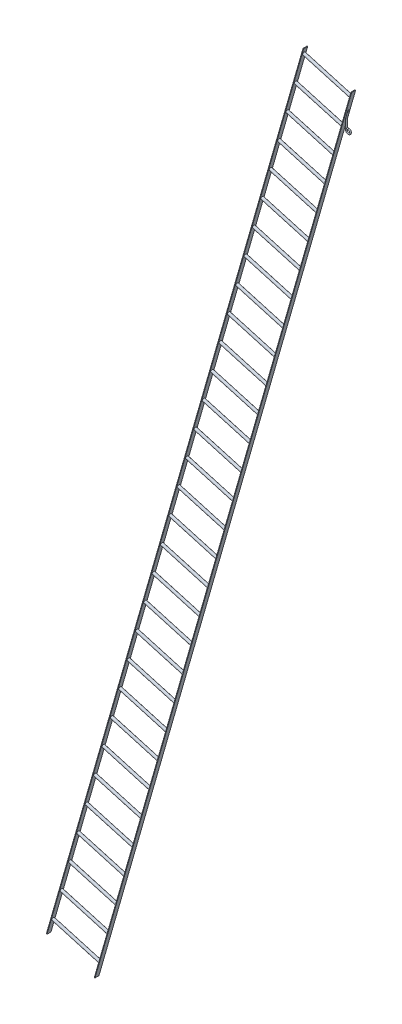
SolidWorks part; units mm, degrees
material "Q235B"
ref_plane "Front Plane" through (0, 0, 0) normal (0, 0, 1) x (1, 0, 0)
ref_plane "Top Plane" through (0, 0, 0) normal (0, 1, 0) x (1, 0, 0)
ref_plane "Right Plane" through (0, 0, 0) normal (1, 0, 0) x (0, 0, -1)
sketch "18 (ProfileFeature) (+7 more in 7 files) Sketch1" plane through (0, 0, 0) normal (0, 0, 1) x (1, 0, 0)
  line L0 (-20, 0) -> (-20, 100.1568)
  line L1 (-19.7676, 101.8106) -> (2.3661, 179)
  line L2 (0, 20) -> (-13.95, 20)
  arc A0 (-20, 0) -> (0, 20) centre (0, 0) ccw
  arc A1 (-20, 100.1568) -> (-19.7676, 101.8106) centre (-14, 100.1568) cw
  point P9 (-20, 101)
  dimension "D1" = 40
  dimension "D6" = 6
  dimension "D2" = 101
  dimension "D3" = 164
  dimension "D4" = 78
  dimension "D5" = 6.05
sweep "Sweep2" add path "18 (ProfileFeature) (+7 more in 7 files) Sketch1" circular profile diameter 12 parameters "D3"=12
chamfer "Chamfer1" distance 0.5 angle 45 1 edges at (-3.4014, 180.6538, 0)
sketch "Sketch2" plane through (0, 0, 0) normal (0, 0, 1) x (1, 0, 0)
  line L0 (56.1154, 366.446) -> (-424.5154, 504.2647) construction
  line L3 (-2488.2722, -8485.1204) -> (50.3479, 368.0999)
  line L4 (-3.5392, 180.1732) -> (-25.5351, 103.4644) construction
  line L5 (-424.5154, 504.2647) -> (-2963.1355, -8348.9555)
  line L6 (-2921.7899, -8204.7663) -> (-2446.9266, -8340.9311)
  line L7 (-2839.0987, -7916.3877) -> (-2364.2354, -8052.5526)
  line L8 (2.3661, 179) -> (56.1154, 366.446)
  line L9 (7.6531, 177.484) -> (-2.9208, 180.516) construction
  dimension "D1" = 9210
  dimension "D2" = 494
  dimension "D3" = 150
  dimension "D4" = 300
  dimension "D5" = 195
ref_plane "Plane2" through (0, 0, -20) normal (0, 0, 1) x (1, 0, 0)
sketch "Sketch7" plane through (0, 0, -20) normal (0, 0, 1) x (1, 0, 0)
  line L0 (-2839.0987, -7916.3877) -> (-2364.2354, -8052.5526) construction
  line L1 (-2921.7899, -8204.7663) -> (-2446.9266, -8340.9311) construction
  line L2 (-424.5154, 504.2647) -> (-2963.1355, -8348.9555) construction
  line L3 (-2488.2722, -8485.1204) -> (50.3479, 368.0999) construction
  line L4 (-2839.0987, -7916.3877) -> (-2364.2354, -8052.5526)
  line L5 (-2921.7899, -8204.7663) -> (-2446.9266, -8340.9311)
  line L6 (-424.5154, 504.2647) -> (-2963.1355, -8348.9555)
  line L7 (-2488.2722, -8485.1204) -> (50.3479, 368.0999)
other "GB/T 704-1988 hot-rolled flat steel 40×6(1)"
ref_plane "Plane3" through (-2488.2722, -8485.1204, -20) normal (-0.2756, -0.9613, 0) x (0, 0, 1)
sketch "Sketch1" plane through (-2488.2722, -8485.1204, -20) normal (-0.2756, -0.9613, 0) x (0, 0, 1)
  line L0 (0, 0) -> (0, 6)
  line L1 (40, 0) -> (40, 6)
  line L3 (0, 6) -> (40, 6)
  line L4 (20, 6) -> (20, 0) construction
  line L5 (40, 0) -> (0, 0)
  point P1 (0, 0)
  point P10 (20, 0)
  point P16 (20, 6)
  point P18 (40, 6)
  dimension "D3" = 40
  dimension "D1" = 6
other "GB/T 6728-2002 round tube 26.8 X 3(2)"
ref_plane "Plane5" through (-2921.7899, -8204.7663, 0) normal (0.9613, -0.2756, 0) x (0.2756, 0.9613, 0)
sketch "Sketch13" plane through (-2921.7899, -8204.7663, 0) normal (0.9613, -0.2756, 0) x (0.2756, 0.9613, 0)
  circle A0 centre (0, 0) radius 10.4
  circle A1 centre (0, 0) radius 13.4
  point P3 (0, 0)
  dimension "Out_dia" = 26.8
  dimension "D1" = 3
  dimension "D2" = 20.8
other "Trim/Extend1"
pattern_linear "LPattern1" count 30 spacing 300 along (0.2756, 0.9613, 0) of bodies 113
